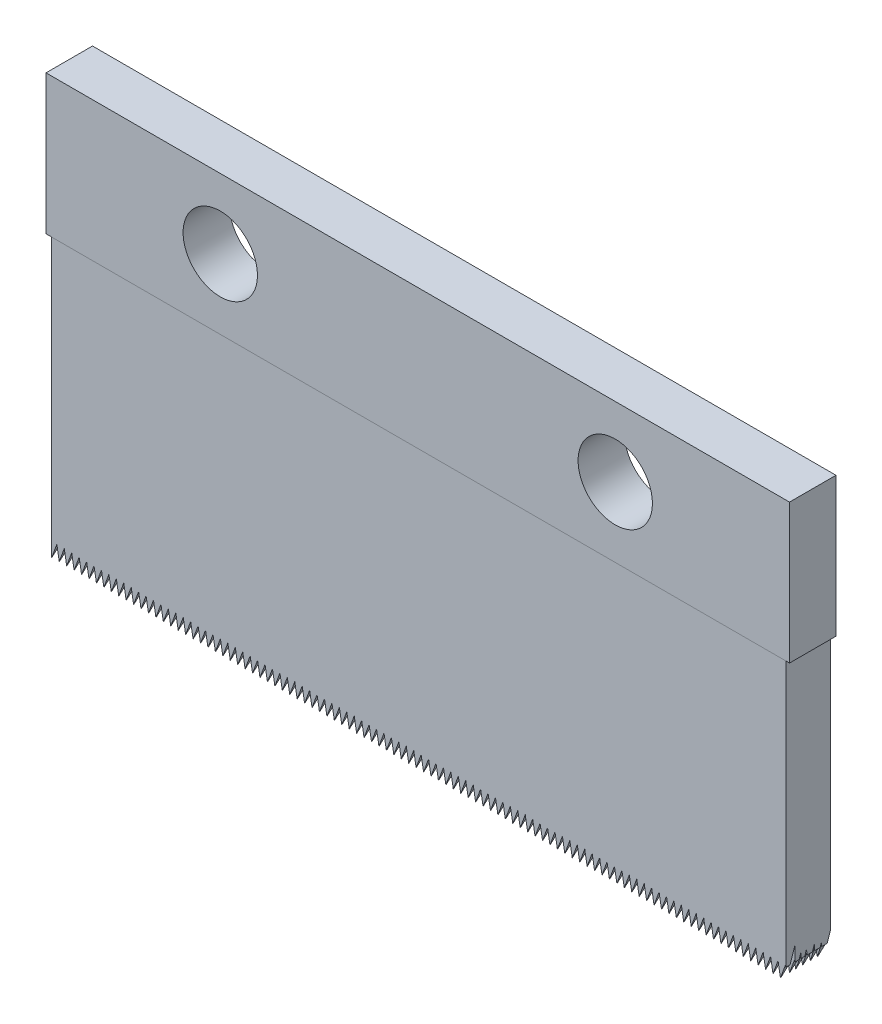
SolidWorks part; units mm, degrees
ref_plane "前视基准面" through (0, 0, 0) normal (0, 0, 1) x (1, 0, 0)
ref_plane "上视基准面" through (0, 0, 0) normal (0, 1, 0) x (1, 0, 0)
ref_plane "右视基准面" through (0, 0, 0) normal (1, 0, 0) x (0, 0, -1)
sketch "草图1" plane through (0, 0, 0) normal (0, 0, 1) x (1, 0, 0)
  line L0 (0, 0) -> (0, 20.2561) construction
  line L1 (40, -7.5) -> (-40, -7.5)
  line L2 (40, -7.5) -> (40, 7.5)
  line L3 (40, 7.5) -> (-40, 7.5)
  line L4 (-40, -7.5) -> (-40, 7.5)
  line L5 (40, -7.5) -> (-40, 7.5) construction
  line L6 (40, 7.5) -> (-40, -7.5) construction
  circle A0 centre (-21.25, 0) radius 4
  circle A1 centre (21.25, 0) radius 4
  point P0 (0, 0)
  dimension "D3" = 42.5
  dimension "D1" = 80
  dimension "D2" = 15
extrude "凸台-拉伸1" add sketch "草图1" along normal blind 5
sketch "草图2" plane through (0, -7.5, 0) normal (0, -1, 0) x (1, 0, 0)
  line L0 (40, 5) -> (40, 0) construction
  line L1 (-39.5, 4.9) -> (39.5, 4.9)
  line L2 (-39.5, 4.9) -> (-39.5, 0.1)
  line L3 (-39.5, 0.1) -> (39.5, 0.1)
  line L4 (39.5, 4.9) -> (39.5, 0.1)
  line L5 (-40, 5) -> (-40, 0) construction
  line L6 (-40, 0) -> (40, 0) construction
  line L7 (-40, 5) -> (40, 5) construction
  dimension "D1" = 0.5
  dimension "D2" = 0.5
  dimension "D3" = 0.1
  dimension "D4" = 0.1
extrude "凸台-拉伸2" add sketch "草图2" along normal blind 30
sketch "草图3" plane through (39.5, 0, 0) normal (1, 0, 0) x (0, 0, -1)
  line L0 (-4.9, -37.5) -> (-3.9199, -34.6117)
  line L1 (-3.9199, -34.6117) -> (-3.9199, -37.5)
  line L2 (-4.9, -37.5) -> (-4.9, -7.5) construction
  line L3 (-3.9199, -37.5) -> (-3.2591, -35.5526)
  line L4 (-3.2591, -35.5526) -> (-3.2591, -37.5)
  line L5 (-3.2591, -37.5) -> (-2.6684, -35.5299)
  line L6 (-2.0836, -39.3237) -> (-4.9, -38.8359)
  line L7 (-4.9, -38.8359) -> (-4.9, -37.5)
  line L9 (-2.6684, -35.5299) -> (-2.5, -37.5)
  line L10 (-2.5, -37.5) -> (-1.8334, -35.5552)
  line L11 (-1.8334, -35.5552) -> (-1.6672, -37.5)
  line L12 (-1.6672, -37.5) -> (-1.0649, -35.7428)
  line L13 (-1.0649, -35.7428) -> (-0.9146, -37.5)
  line L14 (-0.9146, -37.5) -> (-0.1, -35.1233)
  line L16 (-0.1, -35.1233) -> (4.7565, -37.5)
  line L17 (4.7565, -37.5) -> (-2.0836, -39.3237)
  line L18 (-0.1, -37.5) -> (-4.9, -37.5) construction
  line L19 (-0.1, -37.5) -> (-0.1, -7.5) construction
  point P5 (-4.9, -27.5)
  point P9 (0, 0)
  point P15 (0, 0)
  point P19 (-4.9, -36.3304)
  point P20 (-4.9, -37.5)
  point P22 (0, 0)
  point P24 (0, 0)
  point P25 (0, 0)
  point P26 (-0.9339, -25.8649)
  point P27 (0, -25.7028)
  point P29 (-3.9199, -37.5)
  point P30 (-3.2742, -27.5)
  point P31 (-3.2514, -37.5)
  point P34 (-2.5, -37.5)
  point P35 (-0.9162, -37.5)
  point P36 (-1.6672, -37.5)
  point P37 (0, 0)
  point P38 (0, 0)
  point P39 (-4.9, -38.8359)
  point P40 (-2.0836, -39.3237)
  point P41 (4.7565, -37.5)
  point P42 (-0.1, -35.0701)
  point P45 (-2.6684, -35.5552)
  point P46 (-3.2514, -35.5299)
extrude "切除-拉伸1" cut sketch "草图3" against normal blind 90
sketch "草图4" plane through (0, 0, 4.9) normal (0, 0, 1) x (1, 0, 0)
  line L0 (-39.5, -37.5) -> (-38.9351, -35.948)
  line L1 (-38.9351, -35.948) -> (-38.6661, -37.5)
  line L2 (39.5, -37.5) -> (-39.5, -37.5) construction
  line L3 (-38.6661, -37.5) -> (-38.6661, -38.2377)
  line L4 (-38.6661, -38.2377) -> (-39.5, -37.5)
  line L5 (-39.5, -37.5) -> (-39.5, -7.5) construction
  dimension "D1" = 160
  dimension "D2" = 99.833
  dimension "D3" = 141.33
  dimension "D4" = 0.8339
extrude "切除-拉伸2" cut sketch "草图4" against normal blind 90
pattern_linear "阵列(线性)1" count 102 spacing 0.8 along (1, 0, 0) of "切除-拉伸2"
